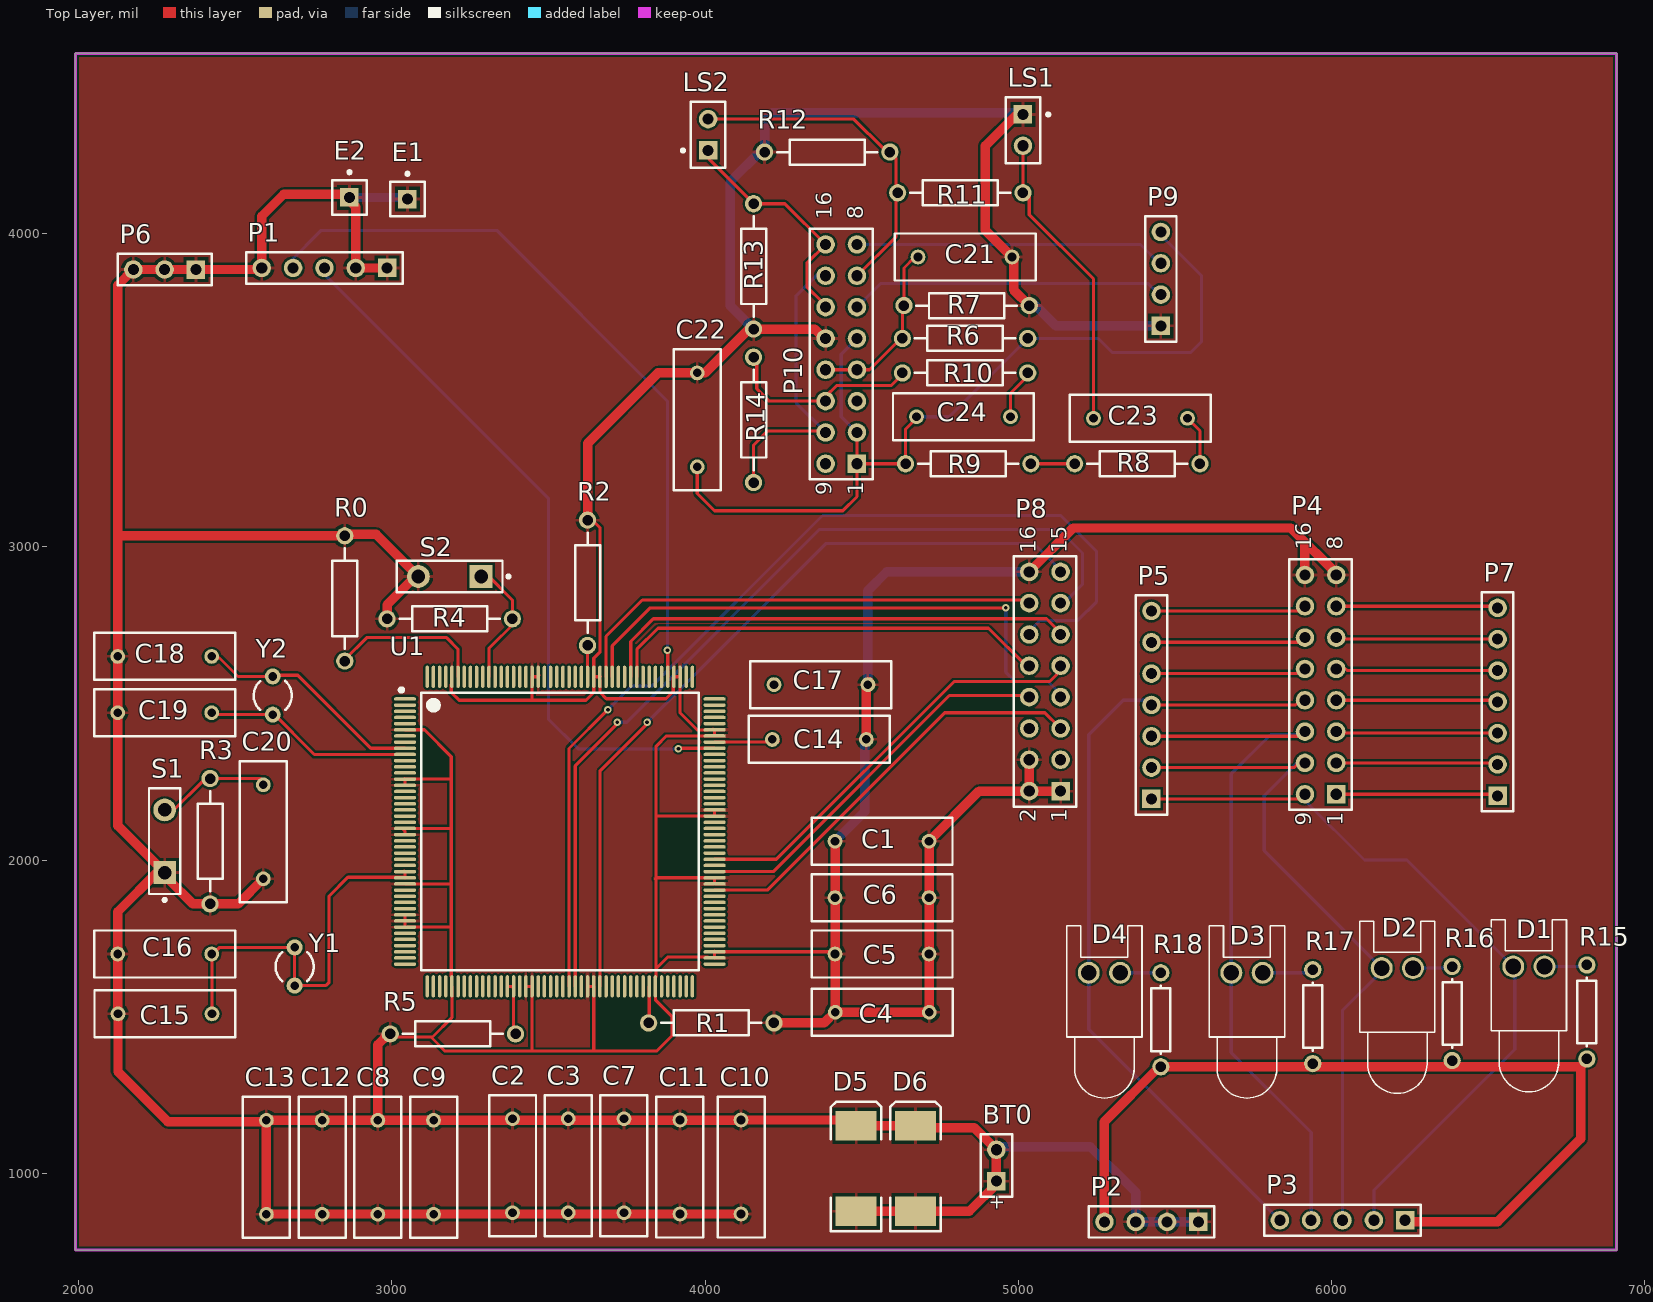
[diagram p0: Top Layer view]
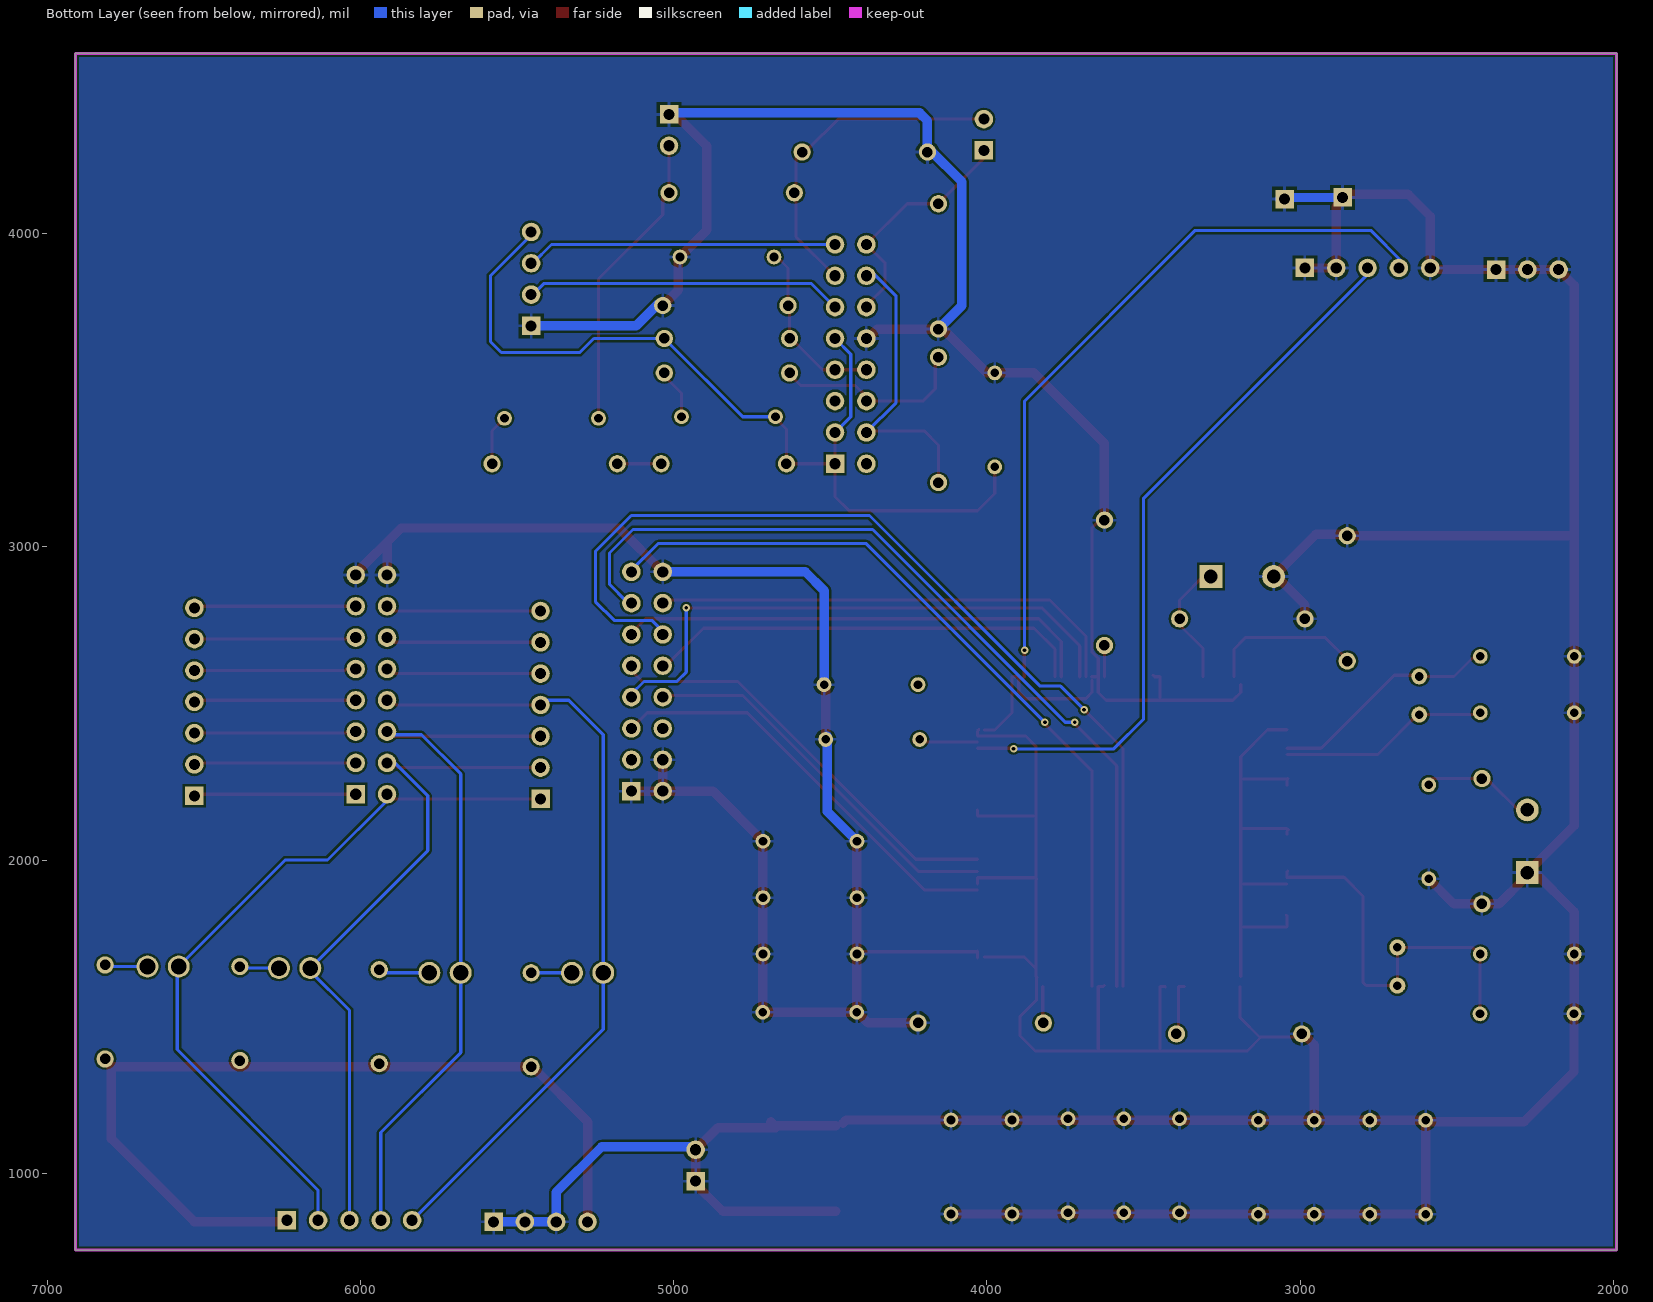
[diagram p1: Bottom Layer view, seen from below]
# Altium PCB MISC80550.PcbDoc
Units mil, origin at the board's own origin, x right, y up, seen from the top; angles counter-clockwise.
Board outline 4920 x 3820 mil, 2 copper layers (Top Layer, Bottom Layer); 69 components, 56 nets, 373 pads, 6 vias.

## Layer stack, top to bottom (the 12.6 mil dielectric is the usual default, probably not edited)
Top Solder: solder mask 0.4, Solder Resist, Dk 3.5
Top Layer: signal copper 1.4
Dielectric1: dielectric 12.6, FR-4, Dk 4.8
Bottom Layer: signal copper 1.4
Bottom Solder: solder mask 0.4, Solder Resist, Dk 3.5

## Board outline
1990,755 1990,4575 6910,4575 6910,755

## Design rules (kind name [scope] priority, off if disabled: settings)
Clearance [All] p1: gap=7
MinimumSolderMaskSliver [All] p1: minsoldermaskwidth=0
PolygonConnect [All] p1: connectstyle=Relief reliefconductorwidth=10 reliefentries=4 polygonreliefangle="90 Angle" airgapwidth=10
RoutingVias [All] p1: holewidth=28 width=50 viastyle="Through Hole" minholewidth=28 minwidth=50 maxholewidth=28 maxwidth=50
SilkToSilkClearance [All] p1: silktosilkclearance=0
SilkToSolderMaskClearance SilkscreenOverComponentPads [IsPad] p1: minsilkscreentomaskgap=0 clearancetoexposedcopper=TRUE
SolderMaskExpansion [All] p1: expansion=4
Width [All] p1: maxlimit=30 minlimit=10 preferedwidth=10
27 further rules are at their usual default settings.

## Components (designator, comment, footprint, x,y, rotation, side; value= is the part's Value field where it differs from the comment)
BT0 "Battery" BAT-2 4930,1025 r90 top
C1 "Cap" RAD-0.3 4565,2060 r180 top
C2 "Cap" RAD-0.3 3385.43,1024.08 r90 top
C3 "Cap" RAD-0.3 3563.31,1024.08 r90 top
C4 "Cap" RAD-0.3 4565.92,1513.94 r180 top
C5 "Cap" RAD-0.3 4565,1700 r180 top
C6 "Cap" RAD-0.3 4565,1880 r180 top
C7 "Cap" RAD-0.3 3741.18,1024.08 r90 top
C8 "Cap" RAD-0.3 2955.55,1019.08 r90 top
C9 "Cap" RAD-0.3 3133.43,1019.08 r90 top
C10 "Cap" RAD-0.3 4115,1020 r90 top
C11 "Cap" RAD-0.3 3920,1020 r90 top
C12 "Cap" RAD-0.3 2777.68,1019.08 r90 top
C13 "Cap" RAD-0.3 2599.8,1019.08 r90 top
C14 "Cap" RAD-0.3 4365,2385 r180 top
C15 "Cap" RAD-0.3 2276.06,1508.9 r0 top
C16 "Cap" RAD-0.3 2275,1700 r0 top
C17 "Cap" RAD-0.3 4370,2560 r180 top
C18 "Cap" RAD-0.3 2275,2650 r0 top
C19 "Cap" RAD-0.3 2275,2470 r0 top
C20 "Cap" RAD-0.3 2590,2090 r90 top
C21 "Cap" RAD-0.3 4830,3925 r180 top
C22 "Cap" RAD-0.3 3975,3405 r270 top
C23 "Cap" RAD-0.3 5390,3410 r0 top
C24 "Cap" RAD-0.3 4825,3415 r180 top
D1 "LED1" LED-0 6630,1660 r0 top
D2 "LED2" LED-0 6210,1655 r0 top
D3 "LED3" LED-0 5730,1640 r0 top
D4 "LED4" LED-0 5275,1640 r0 top
D5 "Diode" DSO-C2/X3.3 4482.2,1015.49 r90 top
D6 "Diode" DSO-C2/X3.3 4671.69,1015.49 r90 top
E1 "Antenna" PIN1 3050,4110 r0 top
E2 "Antenna" PIN1 2865,4115 r0 top
LS1 "Bell" PIN2 5015,4380 r270 top
LS2 "Bell" PIN2 4010,4265 r90 top
P1 "Header 5" HDR1X5 2985,3890 r180 top
P2 "Header 4" HDR1X4 5575,845 r180 top
P3 "Header 5" HDR1X5 6235,850 r180 top
P4 "ULN2003" HDR2X8_CEN 6015,2210 r90 top
P5 "Header 7" HDR1X7 5425,2195 r90 top
P6 "Header 3" HDR1X3 2375,3885 r180 top
P7 "Header 7" HDR1X7 6530,2205 r90 top
P8 "Header 8X2" HDR2X8 5135,2220 r90 top
P9 "CON4" HDR1X4 5455,3705 r90 top
P10 "Header 8X2A" HDR2X8_CEN 4485,3265 r90 top
R0 "Res2" AXIAL-0.4 2850,2835 r90 top
R1 "Res2" AXIAL-0.4 4020,1480 r0 top
R2 "Res2" AXIAL-0.4 3625,2885 r90 top
R3 "Res2" AXIAL-0.4 2420,2060 r270 top
R4 "Res2" AXIAL-0.4 3185,2770 r0 top
R5 "Res2" AXIAL-0.4 3195,1445 r0 top
R6 "Res2" AXIAL-0.4 4830,3665 r180 top
R7 "Res2" AXIAL-0.4 4835,3770 r180 top
R8 "Res2" AXIAL-0.4 5380,3265 r0 top
R9 "Res2" AXIAL-0.4 4840,3265 r0 top
R10 "Res2" AXIAL-0.4 4830,3555 r0 top
R11 "Res2" AXIAL-0.4 4815,4130 r0 top
R12 "Res2" AXIAL-0.4 4390,4260 r0 top
R13 "Res2" AXIAL-0.4 4155,3895 r90 top
R14 "Res2" AXIAL-0.4 4155,3405 r90 top
R15 "Res1" AXIAL-0.3 6815,1515 r270 top
R16 "Res1" AXIAL-0.3 6385,1510 r270 top
R17 "Res1" AXIAL-0.3 5940,1500 r270 top
R18 "Res1" AXIAL-0.3 5455,1490 r270 top
S1 "SW-PB" SPST-2 2275,2060 r90 top
S2 "SW-PB" SPST-2 3185,2905 r180 top
U1 "Component_1" PCBComponent_1 5442.96,3275.43 r270 top
Y1 "XTAL" BCY-W2/D3.1 2690,1660 r0 top
Y2 "XTAL" BCY-W2/D3.1 2620,2525 r180 top

## Footprints (in the part's own frame and the unit in brackets; to place one, negate y for a bottom-side part, rotate by r counter-clockwise, add the part's x,y. Pads: shape width x height; smd on the part's side, far side on the other; paste and mask are expansions set on the pad)
AXIAL-0.3 [mm] "Axial Device, Thru-Hole; 2 Leads; 0.3 in Pin Spacing"
  round 1.4 hole 0.85: 1(-3.81,0) 2(3.81,0)
  silkscreen extent -2.77,-0.76 2.77,0.76
AXIAL-0.4 [mm] "Axial Device, Thru-Hole; 2 Leads; 0.4 in Pin Spacing"
  round 1.4 hole 0.85: 1(-5.08,0) 2(5.08,0)
  silkscreen extent -4.06,-1.02 4.06,1.02
BAT-2 [mm] "Multicell Battery; 2 Leads"
  rect 1.5x1.5 hole 0.9: 1(-1.27,0)
  round 1.5 hole 0.9: 2(1.27,0)
  silkscreen extent -2.54,-1.27 2.54,1.27
BCY-W2/D3.1 [mm] "Crystal, Thru-Hole; 2 Leads; Body 3.1 x 8.2 mm (Dia.xH)"
  round 1.3 hole 0.7: 1(0,1.55) 2(0,-1.55)
  silkscreen extent -1.55,-1.19 1.55,1.17
DSO-C2/X3.3 [mm] "DO-214-AB/SMC; 2 C-Bend Leads; Body 7.9 x 5.9 mm, inc. leads (LxW)"
  rect 2.4x3.3 smd: 1(-3.475,0) 2(3.475,0)
  silkscreen extent -5.07,-2.05 5.43,2.05
HDR1X3 [mm] "Connector; Header; 3 Position"
  rect 1.5x1.5 hole 0.9: 1(0,0)
  round 1.5 hole 0.9: 2(2.54,0) 3(5.08,0)
  silkscreen extent -1.27,-1.27 6.35,1.27
HDR1X4 [mm] "Connector; Header; 4 Position"
  rect 1.5x1.5 hole 0.9: 1(0,0)
  round 1.5 hole 0.9: 2(2.54,0) 3(5.08,0) 4(7.62,0)
  silkscreen extent -1.27,-1.27 8.89,1.27
HDR1X5 [mm] "Connector; Header; 5 Position"
  rect 1.5x1.5 hole 0.9: 1(0,0)
  round 1.5 hole 0.9: 2(2.54,0) 3(5.08,0) 4(7.62,0) 5(10.16,0)
  silkscreen extent -1.27,-1.27 11.43,1.27
HDR1X7 [mm] "Connector; Header; 7 Position"
  rect 1.5x1.5 hole 0.9: 1(0,0)
  round 1.5 hole 0.9: 2(2.54,0) 3(5.08,0) 4(7.62,0) 5(10.16,0) 6(12.7,0) 7(15.24,0)
  silkscreen extent -1.27,-1.27 16.51,1.27
HDR2X8 [mm] "Connector; Header; 8x2 Position"
  rect 1.5x1.5 hole 0.9: 1(0,0)
  round 1.5 hole 0.9: 2(0,2.54) 3(2.54,0) 4(2.54,2.54) 5(5.08,0) 6(5.08,2.54) 7(7.62,0) 8(7.62,2.54) 9(10.16,0) 10(10.16,2.54) 11(12.7,0) 12(12.7,2.54) 13(15.24,0) 14(15.24,2.54) 15(17.78,0) 16(17.78,2.54)
  silkscreen extent -1.27,-1.27 19.05,3.81
HDR2X8_CEN [mm] "Connector; Header; 8x2 Position"
  rect 1.5x1.5 hole 0.9: 1(0,0)
  round 1.5 hole 0.9: 2(2.54,0) 3(5.08,0) 4(7.62,0) 5(10.16,0) 6(12.7,0) 7(15.24,0) 8(17.78,0) 9(0,2.54) 10(2.54,2.54) 11(5.08,2.54) 12(7.62,2.54) 13(10.16,2.54) 14(12.7,2.54) 15(15.24,2.54) 16(17.78,2.54)
  silkscreen extent -1.27,-1.27 19.05,3.81
LED-0 [mil] "Typical INFRARED GaAs LED; 2 Leads"
  round 70 hole 50: 1(50,0) 2(-50,0)
  silkscreen extent -120,-400 120,150
PCBComponent_1 [mm]
  oval 0.28x1.8 smd: 1(19.337,-60.976) 2(19.837,-60.976) 3(20.337,-60.976) 4(20.837,-60.976) 5(21.337,-60.976) 6(21.837,-60.976) 7(22.337,-60.976) 8(22.837,-60.976) 9(23.337,-60.976) 10(23.837,-60.976) 11(24.337,-60.976) 12(24.837,-60.976) 13(25.337,-60.976) 14(25.837,-60.976) 15(26.337,-60.976) 16(26.837,-60.976) 17(27.337,-60.976) 18(27.837,-60.976) 19(28.337,-60.976) 20(28.837,-60.976) 21(29.337,-60.976) 22(29.837,-60.976) 23(30.337,-60.976) 24(30.837,-60.976) 25(31.337,-60.976) 26(31.837,-60.976) 27(32.337,-60.976) 28(32.837,-60.976) 29(33.337,-60.976) 30(33.837,-60.976) 31(34.337,-60.976) 32(34.837,-60.976) 33(35.337,-60.976) 34(35.837,-60.976) 35(36.337,-60.976) 36(36.837,-60.976) 37(37.337,-60.976) 38(37.837,-60.976) 39(38.337,-60.976) 40(38.837,-60.976) 41(39.337,-60.976) 42(39.837,-60.976) 43(40.337,-60.976) 44(40.837,-60.976) 89(40.837,-35.876) 90(40.337,-35.876) 91(39.837,-35.876) 92(39.337,-35.876) 93(38.837,-35.876) 94(38.337,-35.876) 95(37.837,-35.876) 96(37.337,-35.876) 97(36.837,-35.876) 98(36.337,-35.876) 99(35.837,-35.876) 100(35.337,-35.876) 101(34.837,-35.876) 102(34.337,-35.876) 103(33.837,-35.876) 104(33.337,-35.876) 105(32.837,-35.876) 106(32.337,-35.876) 107(31.837,-35.876) 108(31.337,-35.876) 109(30.837,-35.876) 110(30.337,-35.876) 111(29.837,-35.876) 112(29.337,-35.876) 113(28.837,-35.876) 114(28.337,-35.876) 115(27.837,-35.876) 116(27.337,-35.876) 117(26.837,-35.876) 118(26.337,-35.876) 119(25.837,-35.876) 120(25.337,-35.876) 121(24.837,-35.876) 122(24.337,-35.876) 123(23.837,-35.876) 124(23.337,-35.876) 125(22.837,-35.876) 126(22.337,-35.876) 127(21.837,-35.876) 128(21.337,-35.876) 129(20.837,-35.876) 130(20.337,-35.876) 131(19.837,-35.876) 132(19.337,-35.876)
  oval 1.8x0.28 smd: 45(42.637,-59.176) 46(42.637,-58.676) 47(42.637,-58.176) 48(42.637,-57.676) 49(42.637,-57.176) 50(42.637,-56.676) 51(42.637,-56.176) 52(42.637,-55.676) 53(42.637,-55.176) 54(42.637,-54.676) 55(42.637,-54.176) 56(42.637,-53.676) 57(42.637,-53.176) 58(42.637,-52.676) 59(42.637,-52.176) 60(42.637,-51.676) 61(42.637,-51.176) 62(42.637,-50.676) 63(42.637,-50.176) 64(42.637,-49.676) 65(42.637,-49.176) 66(42.637,-48.676) 67(42.637,-48.176) 68(42.637,-47.676) 69(42.637,-47.176) 70(42.637,-46.676) 71(42.637,-46.176) 72(42.637,-45.676) 73(42.637,-45.176) 74(42.637,-44.676) 75(42.637,-44.176) 76(42.637,-43.676) 77(42.637,-43.176) 78(42.637,-42.676) 79(42.637,-42.176) 80(42.637,-41.676) 81(42.637,-41.176) 82(42.637,-40.676) 83(42.637,-40.176) 84(42.637,-39.676) 85(42.637,-39.176) 86(42.637,-38.676) 87(42.637,-38.176) 88(42.637,-37.676) 133(17.537,-37.676) 134(17.537,-38.176) 135(17.537,-38.676) 136(17.537,-39.176) 137(17.537,-39.676) 138(17.537,-40.176) 139(17.537,-40.676) 140(17.537,-41.176) 141(17.537,-41.676) 142(17.537,-42.176) 143(17.537,-42.676) 144(17.537,-43.176) 145(17.537,-43.676) 146(17.537,-44.176) 147(17.537,-44.676) 148(17.537,-45.176) 149(17.537,-45.676) 150(17.537,-46.176) 151(17.537,-46.676) 152(17.537,-47.176) 153(17.537,-47.676) 154(17.537,-48.176) 155(17.537,-48.676) 156(17.537,-49.176) 157(17.537,-49.676) 158(17.537,-50.176) 159(17.537,-50.676) 160(17.537,-51.176) 161(17.537,-51.676) 162(17.537,-52.176) 163(17.537,-52.676) 164(17.537,-53.176) 165(17.537,-53.676) 166(17.537,-54.176) 167(17.537,-54.676) 168(17.537,-55.176) 169(17.537,-55.676) 170(17.537,-56.176) 171(17.537,-56.676) 172(17.537,-57.176) 173(17.537,-57.676) 174(17.537,-58.176) 175(17.537,-58.676) 176(17.537,-59.176)
  silkscreen extent 18.46,-61.42 41.34,-37.18
PIN1 [mm] "Generic Antenna; 1 Lead"
  rect 1.5x1.5 hole 0.9: 1(0,0)
  silkscreen extent -1.4,-1.4 1.4,2.17
PIN2 [mm] "Photosensitive Diode; 2 Leads"
  rect 1.5x1.5 hole 0.9: 1(0,0)
  round 1.5 hole 0.9: 2(2.54,0)
  silkscreen extent -1.4,-1.4 3.94,2.18
RAD-0.3 [mm] "Radial Cap, Thru-Hole; 2 Leads; 0.3 in Pin Spacing"
  round 1.2 hole 0.7: 1(-3.81,0) 2(3.81,0)
  silkscreen extent -5.71,-1.91 5.71,1.91
SPST-2 [mm] "Circuit Breaker; 2 Leads"
  rect 1.85x1.85 hole 1.1: 1(-2.54,0)
  round 1.85 hole 1.1: 2(2.54,0)
  silkscreen extent -4.89,-1.27 4.28,1.27

## Part data
BT0: "Multicell Battery"
C1 C2 C3 C4 C5 C6 C7 C8 C9 C10 C11 C12 C13 C14 C15 C16 C17 C18 C19 C20 C21 C22 C23 C24: "Capacitor"
D1 D2 D3 D4: library part LED0, "Typical INFRARED GaAs LED"
D5 D6: "Default Diode"
E1 E2: "Generic Antenna"
LS1 LS2: "Electrical Bell"
P1 P3: "Header, 5-Pin"
P2: "Header, 4-Pin"
P4: library part "Header 8X2A", "ULN2003, Dual row"
P5 P7: "Header, 7-Pin"
P6: "Header, 3-Pin"
P8 P10: "Header, 8-Pin, Dual row"
P9: library part "Header 4", "Header, 4-Pin"
R0 R1 R2 R3 R4 R5 R6 R7 R8 R9 R10 R11 R12 R13 R14 R15 R16 R17 R18: "Resistor"
S1 S2: "Switch"
Y1 Y2: "Crystal Oscillator"

## Via types
v1: diameter 24, hole 12, Top Layer to Bottom Layer, 6 vias

## Nets (pads, with @x,y where several pads share a name; then routed paths per layer and width w, separated by ;. In a path a pad name is that pad's centre, name@x,y a point inside that pad or via, vN(x,y) a via of type N, cw(c..) or ccw(c..) an arc to the next point about the centre after c; other vN are vias at no path point)
1B: P4.1 P7.1 | length 544.1
  Top Layer w10: P4.1 6545,2210 P7.1@6555,2200
1C: D1.2 P3.2 P4.9 P5.1 | length 2386.3
  Top Layer w10: P5.1 5900,2195 P4.9 P4.9@5925,2220
  Bottom Layer w10: P4.9@5915,2190 6105,2000 6240,2000 D1.2 ; P3.2 6135,945 6585,1395 D1.2@6585,1655
2B: P4.2 P7.2 | length 533.3
  Top Layer w10: P4.2 6520,2310 P7.2@6540,2290
2C: D2.2 P3.3 P4.10 P5.2 | length 2183.9
  Top Layer w10: P5.2 5880,2295 P4.10@5895,2310
  Bottom Layer w10: P4.10@5890,2310 5785,2205 5785,2030 D2.2 ; P3.3 6035,1520 D2.2@6165,1650
3B: P4.3 P7.3 | length 510
  Top Layer w10: P4.3@6020,2405 P7.3
3C: D3.2 P3.4 P4.11 P5.3 | length 2284.5
  Top Layer w10: P5.3 5910,2395 P4.11@5915,2400
  Bottom Layer w10: D3.2@5680,1630 5680,1385 5935,1130 P3.4 ; D3.2 5680,2275 5805,2400 P4.11@5900,2400
4B: P4.4 P7.4 | length 517.1
  Top Layer w10: P4.4 6525,2510 P7.4
4C: D4.2 P3.5 P4.12 P5.4 | length 2541.5
  Top Layer w10: P5.4 5885,2495 P4.12@5905,2515
  Bottom Layer w10: P5.4@5430,2510 5335,2510 5225,2400 D4.2 5225,1460 P3.5
5B: P4.5 P7.5 | length 507.1
  Top Layer w10: P4.5@6025,2610 6045,2610 6050,2605 P7.5
5C: P4.13 P5.5 | length 493.3
  Top Layer w10: P5.5 5890,2595 P4.13@5910,2615
6B: P4.6 P7.6 | length 502.1
  Top Layer w10: P4.6@6030,2710 6035,2705 P7.6
6C: P4.14 P5.6 | length 484.1
  Top Layer w10: P5.6 5895,2695 P4.14@5905,2705
7B: P4.7 P7.7 | length 507.1
  Top Layer w10: P4.7 6515,2810 P7.7@6520,2805
7C: P4.15 P5.7 | length 506.2
  Top Layer w10: P5.7 5910,2795 P4.15@5925,2810
BAT_CR1220: BT0.1 BT0.2 C1.1 C1.2 C2.1 C2.2 C3.1 C3.2 C4.1 C4.2 C5.1 C5.2 C6.1 C6.2 C7.1 C7.2 C8.1 C8.2 C9.1 C9.2 C10.1 C10.2 C11.1 C11.2 C12.1 C12.2 C13.1 C13.2 C14.1 C15.1 C16.1 C17.1 C18.1 C19.1 C20.1 C21.1 C22.1 D5.1 D5.2 D6.1 D6.2 E1.1 E2.1 LS1.1 P1.1 P1.2 P1.5 P2.1 P2.2 P2.3 P4.8 P4.16 P6.1 P6.2 P6.3 P8.1 P8.2 P8.4 P8.16 P9.1 P10.13 R0.2 R1.2 R2.2 R3.2 R4.1 R5.1 R7.1 R12.1 R13.1 S1.1 S2.2 U1.6 U1.14 U1.15 U1.22 U1.23 U1.31 U1.36 U1.37 U1.38 U1.49 U1.61 U1.62 U1.71 U1.72 U1.82 U1.90 U1.91 U1.102 U1.103 U1.113 U1.114 U1.126 U1.127 U1.135 U1.136 U1.148 U1.149 U1.158 U1.159 U1.172 | length 27860.6
  Top Layer w10: R5.1@3010,1435 3125,1435 ; U1.22@3038.29,2096.71 3042.33,2092.67 U1.23 ; U1.14@3040,2260 3042.33,2257.67 U1.15 ; U1.31 3188.59,1923.59 3190,1925 ; U1.22 3189.25,2100.75 3190,2100 ; U1.14 3188.23,2258.23 3190,2260 ; U1.6 3104.29,2415.71 3190,2330 3190,2260 ; U1.36@3045,1825 3042.33,1822.33 U1.37 U1.38 3189.21,1785.79 3190,1785 ; U1.49@3190,1629.11 3190,1785 ; U1.172@3190,2560 3190,2535 3215,2510 3445,2510 ; U1.49 3191.93,1496.93 3130,1435 3125,1435 ; U1.61@3430,1595 3431.82,1596.82 U1.62 3447.84,1392.16 3450,1390 ; U1.158@3469.7,2590 3464.7,2585 U1.159 3447.84,2512.84 3445,2510 ; U1.71@3625,1600 3628.18,1596.82 U1.72 3644.69,1395.31 3650,1390 ; R2.2@3625,3100 3665,3060 3665,2665 3644.69,2644.69 U1.149 ; U1.148@3665,2575 3665,2535 3685,2515 3875.38,2515 3898.42,2538.05 3898.42,2582.83 U1.136 3915,2585 U1.135@3920,2580 ; U1.148@3666.55,2585 U1.148 U1.149 ; U1.82@3840,1625 U1.82@3841.54,1626.54 ; 3840,1940 3843.27,1943.27 3843.71,1943.27 ; 3845,2140 3845.12,2140.12 U1.113 4030.51,2159.49 U1.114@4030,2160 ; U1.135 3920.28,2469.72 3975,2415 U1.127@4010,2415 ; U1.90@4010,1690 3880,1690 3843.71,1653.71 ; U1.127@4025,2417.89 4030.51,2412.38 U1.126 3876.03,2396.03 3843.71,2363.71 3843.71,1943.27 ; U1.91@4030,1709.23 4030.51,1708.72 U1.91 ; U1.103@4030,1940 4030.51,1939.49 U1.102 ; U1.90 U1.91 ; U1.103 3843.71,1943.27 ; C5.2@4410,1705 4407.95,1707.05 U1.91 ; 3125,1435 3170,1390 3450,1390 ; 3190,1785 3190,1925 ; 3190,1925 3190,2100 ; 3190,2100 3190,2260 ; 3445,2510 3620,2510 3644.69,2534.69 U1.149 ; 3450,1390 3650,1390 ; 3650,1390 3845,1390 3895,1440 3895,1500 3841.54,1553.46 U1.82 U1.82@3841.54,1626.54 ; U1.82@3841.54,1626.54 3843.71,1628.71 3843.71,1653.71 ; 3843.71,1653.71 3843.71,1943.27
  Top Layer w30: S1.1@2255,1965 2125,1835 C16.1 2125,1505 2126.06,1503.94 2126.06,1323.94 2285,1165 C13.2@2605,1165 ; S1.1 2125,2110 C19.1 C18.1 2125,3035 ; S1.1@2285,1940 2365,1860 R3.2 2510,1860 C20.1 ; C13.1 C13.1@2599.8,870 ; C13.2@2610,1170 C13.2@2609.08,1169.08 ; R0.2 2125,3035 ; R0.2@2865,3040 2950,3040 S2.2@3080,2910 ; E2.1@2865,4105 2885,4085 P1.2 P1.1 ; E2.1@2870,4125 2655,4125 2585,4055 P1.5 2580,3885 P6.1 P6.2 P6.3 2125,3835 2125,3035 ; R4.1 2985,2815 S2.2@3080,2910 ; R5.1@2990,1445 2955.55,1410.55 C8.2 ; S2.2 S2.2@3080,2910 ; R2.2 3625,3100 3625,3330 3850,3555 C22.1 4000,3555 R13.1@4140,3695 ; C10.1 C11.1 C13.1@2599.8,870 ; C10.2 C10.2@4120,1170 ; R13.1 4350,3695 P10.13@4380,3665 ; R1.2 4380,1480 C4.2@4415.92,1515.92 ; C4.2@4420,1520 C4.2@4415.92,1515.92 ; C1.2@4420,2065 4415.92,2060.92 4415.92,1880 C4.2@4415.92,1515.92 ; D5.2@4460,1160 4450,1170 C10.2@4120,1170 ; D5.1 D6.1 4843.68,878.68 BT0.1@4935,970 ; D5.2 D6.2 4677.3,1152.3 D6.2@4690,1165 ; C14.1 4515,2560 C17.1@4525,2570 ; D6.2@4675,1145 4860,1145 BT0.2 ; C1.1 4875,2220 P8.2 ; C1.1@4720,2060 4715.92,2055.92 C4.1 C4.2 C4.2@4415.92,1515.92 ; BT0.1 BT0.2@4930,1070 ; C21.1 4895,4010 4895,4280 LS1.1@5010,4395 ; C21.1@4985,3930 4985,3820 R7.1 ; P8.16 5175,3060 5870,3060 P4.8@6025,2905 ; P8.4@5045,2310 5035,2300 P8.2 ; P8.1@5130,2220 P8.2 ; P4.16 5915,3010 ; C13.1@2599.8,870 2599.8,1159.8 C13.2@2605,1165 ; C13.2@2605,1165 C13.2@2609.08,1169.08 ; C13.2@2609.08,1169.08 C12.2 C8.2 ; C8.2 C9.2 4119.08,1169.08 C10.2@4120,1170
  Bottom Layer w30: E2.1 3060,4115 E1.1@3065,4110 ; R13.1 4080,3770 4080,4165 R12.1@4180,4265 ; R12.1 4190,4360 4215,4385 LS1.1@5015,4385 ; C1.2 4510,2155 C14.1@4510,2395 ; C17.1 4520,2860 4580,2920 P8.16 P8.16@5040,2920 ; BT0.2@4945,1085 5230,1085 5375,940 P2.3 P2.2 5565,845 P2.1@5570,840 ; R7.1@5050,3775 5120,3705 P9.1
BOOT0: R4.2 S2.1 U1.166 | length 390.4
  Top Layer w10: S2.1@3300,2915 3385,2830 R4.2 ; U1.166 3310.04,2675.04 R4.2@3395,2760
ECHO_TX_SDA: P9.2 P10.6 | length 1010.6
  Bottom Layer w10: P10.6 4560,3840 5415,3840 P9.2@5450,3805
FSMC_NE4_B: P8.3
JTCK-SWCLK: P1.4 U1.137 | length 2356.3
  Top Layer w10: U1.137 v1@3880.91,2674.09
  Bottom Layer w10: P1.4@2675,3910 2775,4010 3335,4010 3880,3465 v1(3880,2670)
JTMS-SWDIO: P1.3 U1.124 | length 2284.4
  Top Layer w10: v1@3916.66,2356.66 U1.124
  Bottom Layer w10: P1.3@2785,3870 3500,3155 3500,2450 3595,2355 v1(3915,2355)
NetC14_2: C14.2 U1.125 | length 206
  Top Layer w10: U1.125 4231.34,2376.34 C14.2@4235,2380
NetC20_2: C20.2 R3.1 S1.2 | length 338.5
  Top Layer w10: S1.2 2305,2160 R3.1@2395,2250 ; R3.1 2580,2260 C20.2@2595,2245
NetC21_2: C21.2 P10.4 P10.12 R6.2 R7.2 | length 548
  Top Layer w10: P10.12 P10.4 4525,3565 R6.2@4620,3660 ; R6.2 4630,3755 R7.2@4640,3765 ; R7.2 4635,3890 C21.2@4670,3925
NetC22_2: C22.2 C24.2 P9.4 P10.1 P10.2 P10.5 R6.1 R9.1 | length 2922.9
  Top Layer w10: C22.2 3975,3170 4030,3115 4440,3115 4485,3160 P10.1@4485,3250 ; P10.2@4490,3370 P10.2 P10.1 R9.1 4640,3375 C24.2@4680,3415
  Bottom Layer w10: P10.2@4480,3370 4435,3415 4435,3615 P10.5 ; C24.2 4780,3415 R6.1@5020,3655 ; R6.1 5255,3665 5300,3620 5550,3620 5585,3655 5585,3865 P9.4@5450,4000
NetC23_1: C23.1 LS1.2 R11.2 | length 998.2
  Top Layer w10: LS1.2@5010,4295 5015,4290 LS1.2 R11.2 ; R11.2@5020,4150 5035,4135 5035,4060 5240,3855 C23.1
NetC23_2: C23.2 R8.2 | length 161.6
  Top Layer w10: C23.2 5580,3370 R8.2
NetC24_1: C24.1 R10.2 | length 159.9
  Top Layer w10: C24.1 4975,3490 R10.2@5035,3550
NetD1_1: D1.1 R15.1 | length 141.2
  Bottom Layer w10: D1.1 6800,1660 R15.1@6815,1675
NetD2_1: D2.1 R16.1 | length 100
  Bottom Layer w10: D2.1 R16.1@6360,1655
NetD3_1: D3.1 R17.1 | length 182.1
  Bottom Layer w10: D3.1 5955,1640 R17.1@5960,1645
NetD4_1: D4.1 R18.1 | length 130
  Bottom Layer w10: D4.1 R18.1
NetLS2_1: LS2.1 P10.14 P10.16 R13.2 | length 741.5
  Top Layer w10: LS2.1@4005,4265 4005,4245 R13.2 ; R13.2@4160,4095 4255,4095 P10.16 4325,3905 4325,3830 P10.14@4375,3780
NetLS2_2: LS2.2 P10.7 R11.1 R12.2 | length 1044.4
  Top Layer w10: LS2.2 4475,4365 R12.2@4570,4270 ; P10.7 4610,3990 R11.1@4610,4120 ; R12.2 4610,4240 R11.1@4610,4130
NetP10_10: P10.10 P10.15 R14.1 | length 982
  Top Layer w10: R14.1 4155,3325 4200,3370 P10.10@4400,3370
  Bottom Layer w10: P10.10 4290,3460 4290,3800 4360,3870 P10.15@4385,3870
NetP10_11: P10.11 R10.1 R14.2 | length 637.6
  Top Layer w10: R14.2@4165,3610 4165,3505 4205,3465 P10.11 4385,3480 4420,3515 4595,3515 R10.1@4635,3555
NetR0_1: R0.1 U1.171 | length 494.2
  Top Layer w10: R0.1@2850,2640 2920,2710 3175,2710 3211.62,2673.38 U1.171
NetR1_1: R1.1 U1.81 | length 102.6
  Top Layer w10: R1.1@3820,1495 3821.85,1496.85 U1.81
NetR2_1: R2.1 U1.150 | length 95
  Top Layer w10: U1.150 R2.1@3625,2680
NetR8_1: R8.1 R9.2 | length 144.1
  Top Layer w10: R9.2 5170,3265 R8.1@5180,3275
PB2-BOOT1/RS485_TXEN: R5.2 U1.58 U1.59 | length 165.4
  Top Layer w10: U1.58 3383.18,1596.82 U1.59@3385.98,1594.02 ; U1.59 3388.78,1451.22 R5.2@3390,1450
PC14-OSC32_IN: C18.2 U1.9 Y2.2 | length 723.4
  Top Layer w10: C18.2@2430,2645 2450,2645 2508.98,2586.02 Y2.2 ; Y2.2@2630,2590 2700,2590 2933.34,2356.66 U1.9
PC15-OSC32_OUT: C19.2 U1.10 Y2.1 | length 681.2
  Top Layer w10: C19.2@2425,2460 2428.98,2463.98 Y2.1 ; Y2.1@2615,2475 2753.03,2336.97 U1.10
PD0/FSMC_D2: P8.10 U1.142 | length 1407.7
  Top Layer w10: U1.142 3782.48,2672.48 3850,2740 4905,2740 P8.10@5025,2620
PD1/FSMC_D3: P8.11 U1.143 | length 1526.5
  Top Layer w10: U1.143 3762.8,2697.8 3835,2770 5090,2770 P8.11@5130,2730
PD4/FSMC_NOE: P8.7 U1.146 | length 1814.2
  Top Layer w10: U1.146 3703.74,2683.74 3825,2805 v1(4960,2805)
  Bottom Layer w10: v1(4960,2805) 4960,2600 4990,2570 5095,2570 P8.7@5135,2530
PD5/FSMC_NWE: P8.14 U1.147 | length 1538
  Top Layer w10: U1.147 3684.06,2714.06 3800,2830 P8.14@5045,2830
PD13/FSMC_A18: P8.5 U1.101 | length 1352.6
  Top Layer w10: U1.101 4198.9,1903.9 4765,2470 5085,2470 P8.5@5130,2425
PD14/FSMC_D0: P8.8 U1.104 | length 1232.3
  Top Layer w10: U1.104 4217.96,1962.96 4780,2525 P8.8@5030,2525
PD15/FSMC_D1: P8.9 U1.106 | length 1368.3
  Top Layer w10: U1.106 4227.33,2002.33 4795,2570 5100,2570 P8.9@5145,2615
PE7/FSMC_D4: P8.12 U1.68 | length 3209.8
  Top Layer w10: U1.68 3565.95,2355.95 v1(3690,2480) v1@3692.5,2482.5
  Bottom Layer w10: v1(3690,2480) 3765,2555 3830,2555 4375,3100 5135,3100 5250,2985 5250,2825 5190,2765 5070,2765 P8.12@5040,2735
PE8/FSMC_D5: P8.13 U1.69 | length 2849.5
  Top Layer w10: U1.69 3585.63,2300.63 v1@3725,2440
  Bottom Layer w10: v1(3720,2440) 3750,2440 4365,3055 5130,3055 5205,2980 5205,2880 P8.13@5150,2825
PE9/FSMC_D6: U1.70
PE10/FSMC_D7: P8.15 U1.73 | length 2506
  Top Layer w10: U1.73 3664.37,2199.37 3665,2200 3665,2285 v1@3820,2440
  Bottom Layer w10: v1(3815,2440) 4385,3010 5050,3010 P8.15@5140,2920
PH0-OSC_IN: C15.2 C16.2 U1.29 U1.30 Y1.1 Y1.2 | length 1240.5
  Top Layer w10: C16.2@2420,1690 2426.06,1683.94 C15.2 ; C16.2@2435,1705 2451.02,1721.02 Y1.1 ; Y1.1@2685,1715 2690,1710 Y1.2 2788.98,1598.98 2800,1610 2800,1885 2860,1945 U1.30@3040,1945 ; U1.29@3040,1965 3042.33,1962.67 U1.30
TRIG——RX_SCL_I/O: P9.3 P10.8 | length 989.9
  Bottom Layer w10: P10.8 5390,3965 P9.3@5450,3905
VCC#: P2.4 P3.1 R15.2 R16.2 R17.2 R18.2 | length 2859.7
  Top Layer w30: P2.4 5275,1165 R18.2@5450,1340 ; R18.2 6385,1340 R16.2@6385,1345 ; P3.1 6240,845 6530,845 6795,1110 6795,1340 ; R16.2 R16.2@6385,1345 ; R15.2@6815,1360 6795,1340 ; R16.2@6385,1345 6390,1340 6795,1340
pads on no net: C17.2 P8.6 P10.3 P10.9 U1.1 U1.2 U1.3 U1.4 U1.5 U1.7 U1.8 U1.11 U1.12 U1.13 U1.16 U1.17 U1.18 U1.19 U1.20 U1.21 U1.24 U1.25 U1.26 U1.27 U1.28 U1.32 U1.33 U1.34 U1.35 U1.39 U1.40 U1.41 U1.42 U1.43 U1.44 U1.45 U1.46 U1.47 U1.48 U1.50 U1.51 U1.52 U1.53 U1.54 U1.55 U1.56 U1.57 U1.60 U1.63 U1.64 U1.65 U1.66 U1.67 U1.74 U1.75 U1.76 U1.77 U1.78 U1.79 U1.80 U1.83 U1.84 U1.85 U1.86 U1.87 U1.88 U1.89 U1.92 U1.93 U1.94 U1.95 U1.96 U1.97 U1.98 U1.99 U1.100 U1.105 U1.107 U1.108 U1.109 U1.110 U1.111 U1.112 U1.115 U1.116 U1.117 U1.118 U1.119 U1.120 U1.121 U1.122 U1.123 U1.128 U1.129 U1.130 U1.131 U1.132 U1.133 U1.134 U1.138 U1.139 U1.140 U1.141 U1.144 U1.145 U1.151 U1.152 U1.153 U1.154 U1.155 U1.156 U1.157 U1.160 U1.161 U1.162 U1.163 U1.164 U1.165 U1.167 U1.168 U1.169 U1.170 U1.173 U1.174 U1.175 U1.176

## Polygon pours and split planes (outlines as drawn)
BAT_CR1220 on Bottom Layer "D" (solid, remove dead copper, pour order 0): 1715,4780 1795,4860 7485,4860 7485,990 7005,510 6990,495 1445,495
BAT_CR1220 on Top Layer "D" (solid, remove dead copper, pour order 2): 1740,4750 7550,4750 7580,4720 7165,4305 7165,455 2065,455 1845,675

## Keep-outs
Keep-Out Layer:
  lines w10: 1990,755 1990,4575 6910,4575 6910,755 2485,755 1990,755